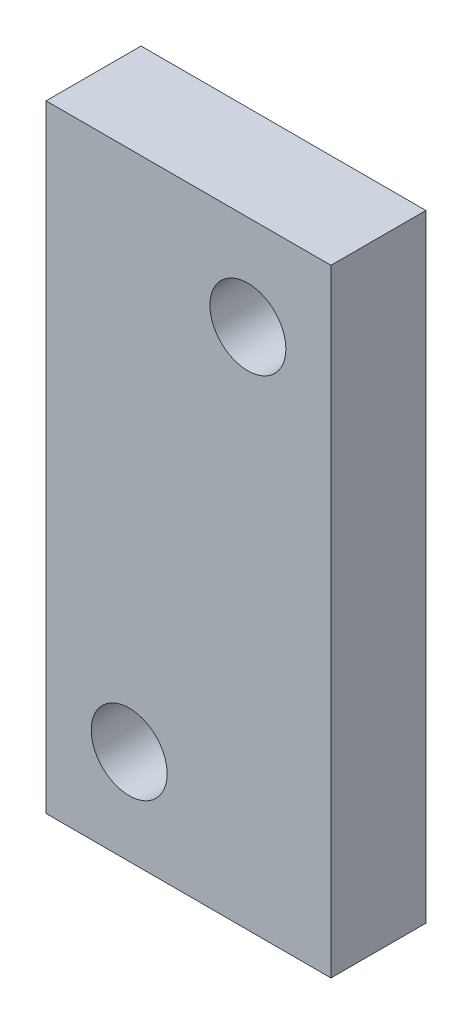
SolidWorks part; units mm, degrees
ref_plane "前视基准面" through (0, 0, 0) normal (0, 0, 1) x (1, 0, 0)
ref_plane "上视基准面" through (0, 0, 0) normal (0, 1, 0) x (1, 0, 0)
ref_plane "右视基准面" through (0, 0, 0) normal (1, 0, 0) x (0, 0, -1)
other "Configuration Table"
sketch "草图1" plane through (0, 0, 0) normal (0, 0, 1) x (1, 0, 0)
  line L0 (-12, -26) -> (12, -26)
  line L1 (12, -26) -> (12, 26)
  line L2 (12, 26) -> (-12, 26)
  line L3 (-12, 26) -> (-12, -26)
  point P0 (0, 0)
  dimension "D1" = 12
  dimension "D2" = 24
  dimension "D3" = 26
  dimension "D4" = 52
extrude "凸台-拉伸1" add sketch "草图1" against normal mid plane 8
sketch "草图2" plane through (0, 0, 0) normal (0, 0, 1) x (1, 0, 0)
  circle A0 centre (-5, -18) radius 3.2
  circle A1 centre (5, 18) radius 3.2
  point P0 (0, 0)
  dimension "D1" = 6.4
  dimension "D2" = 6.4
  dimension "D3" = 5
  dimension "D4" = 10
  dimension "D5" = 18
  dimension "D6" = 36
extrude "切除-拉伸1" cut sketch "草图2" against normal mid plane 28
